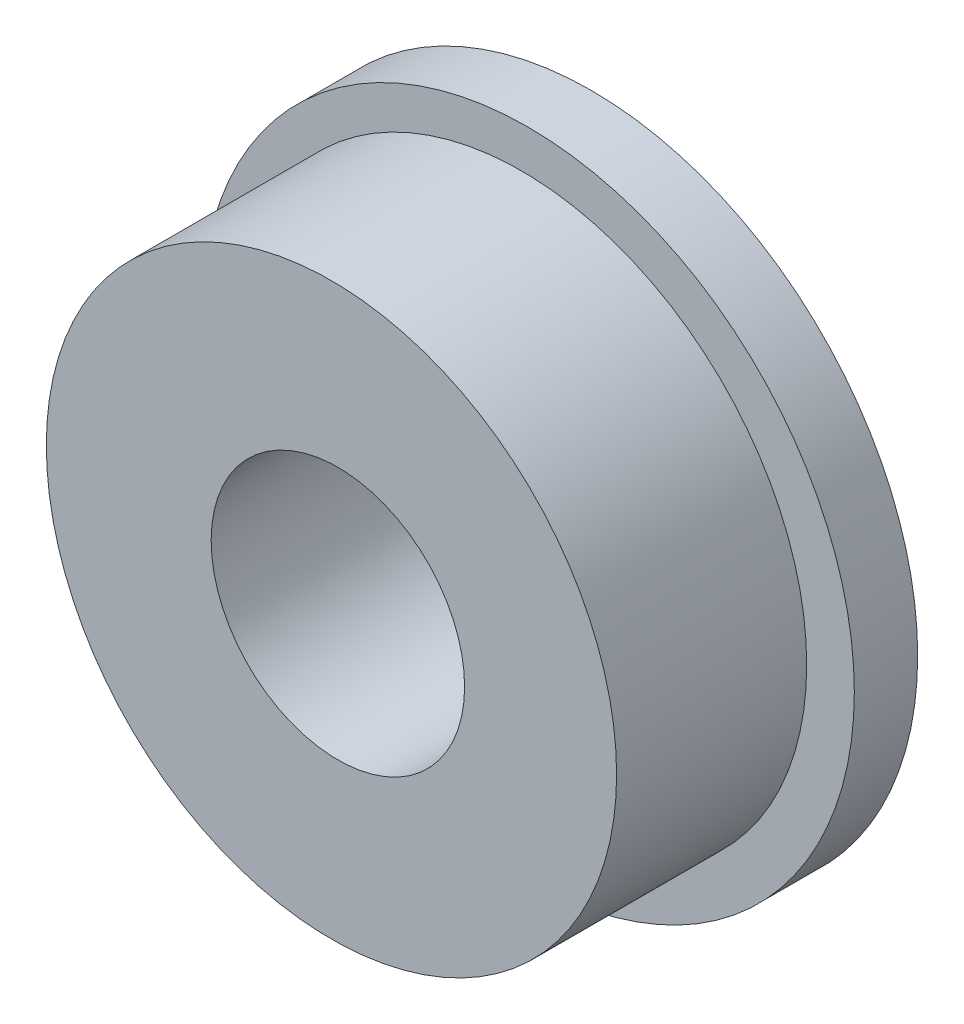
SolidWorks part; units mm, degrees
ref_plane "前视基准面" through (0, 0, 0) normal (0, 0, 1) x (1, 0, 0)
ref_plane "上视基准面" through (0, 0, 0) normal (0, 1, 0) x (1, 0, 0)
ref_plane "右视基准面" through (0, 0, 0) normal (1, 0, 0) x (0, 0, -1)
sketch "草图1" plane through (0, 0, 0) normal (0, 0, 1) x (1, 0, 0)
  circle A0 centre (0, 0) radius 5.15
  circle A1 centre (0, 0) radius 2
  dimension "D1" = 10.3
  dimension "D2" = 4
extrude "凸台-拉伸1" add sketch "草图1" along normal blind 4
sketch "草图2" plane through (0, 0, 4) normal (0, 0, 1) x (1, 0, 0)
  circle A0 centre (0, 0) radius 5.15
  circle A1 centre (-0.1013, 0) radius 4.5
  dimension "D1" = 9
extrude "切除-拉伸1" cut sketch "草图2" against normal blind 3
